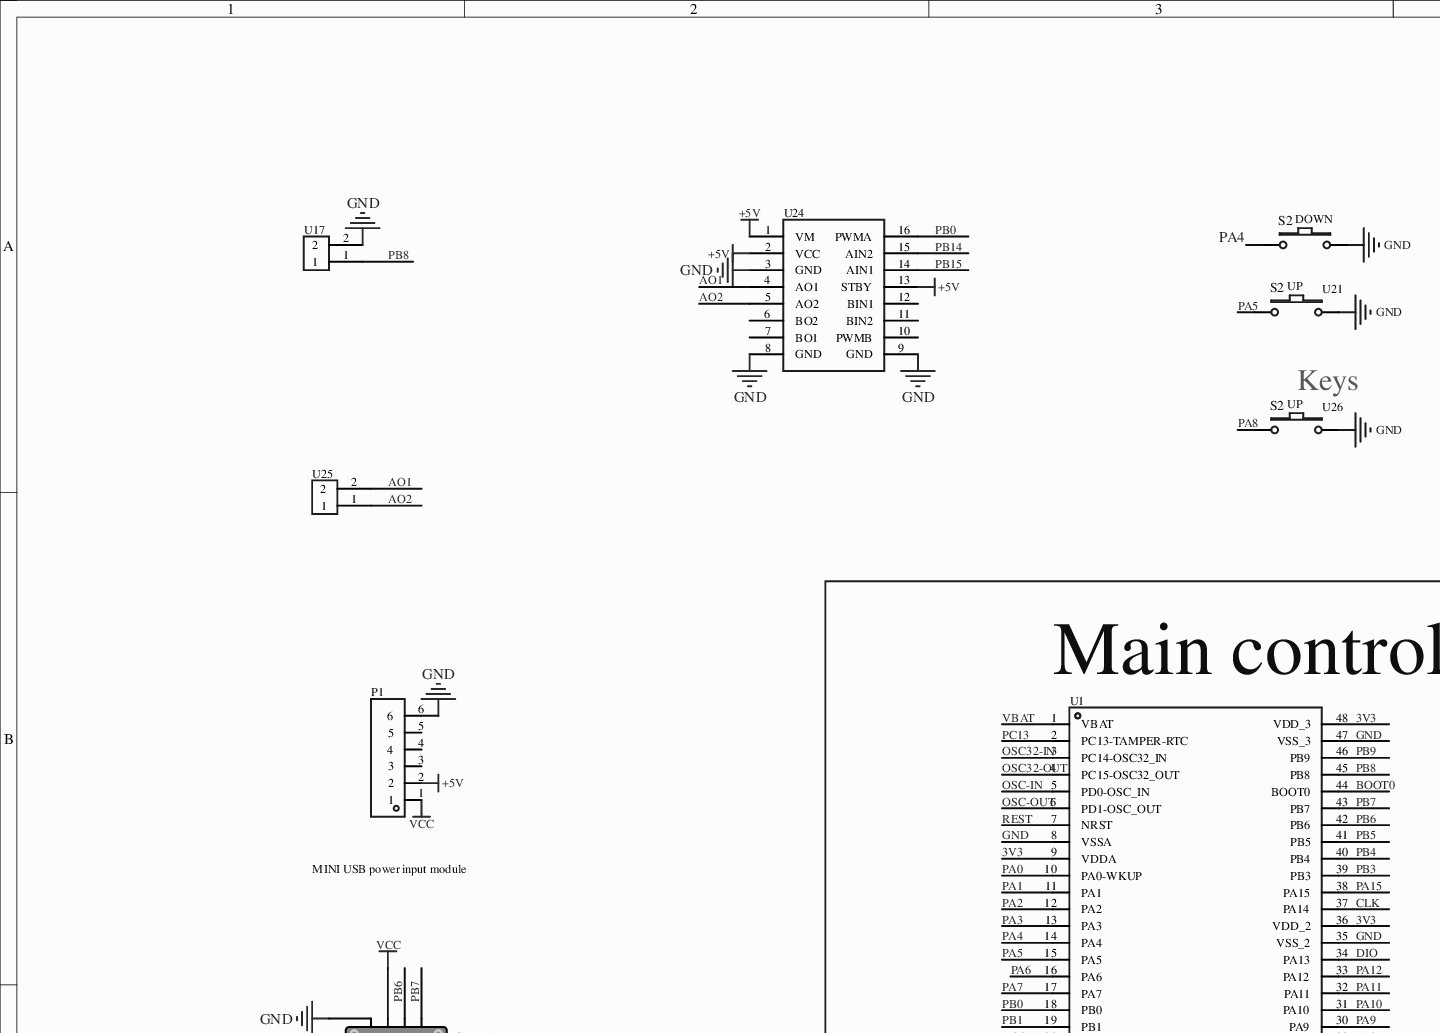
[diagram p0: MISC89131-3.schdoc, top left]
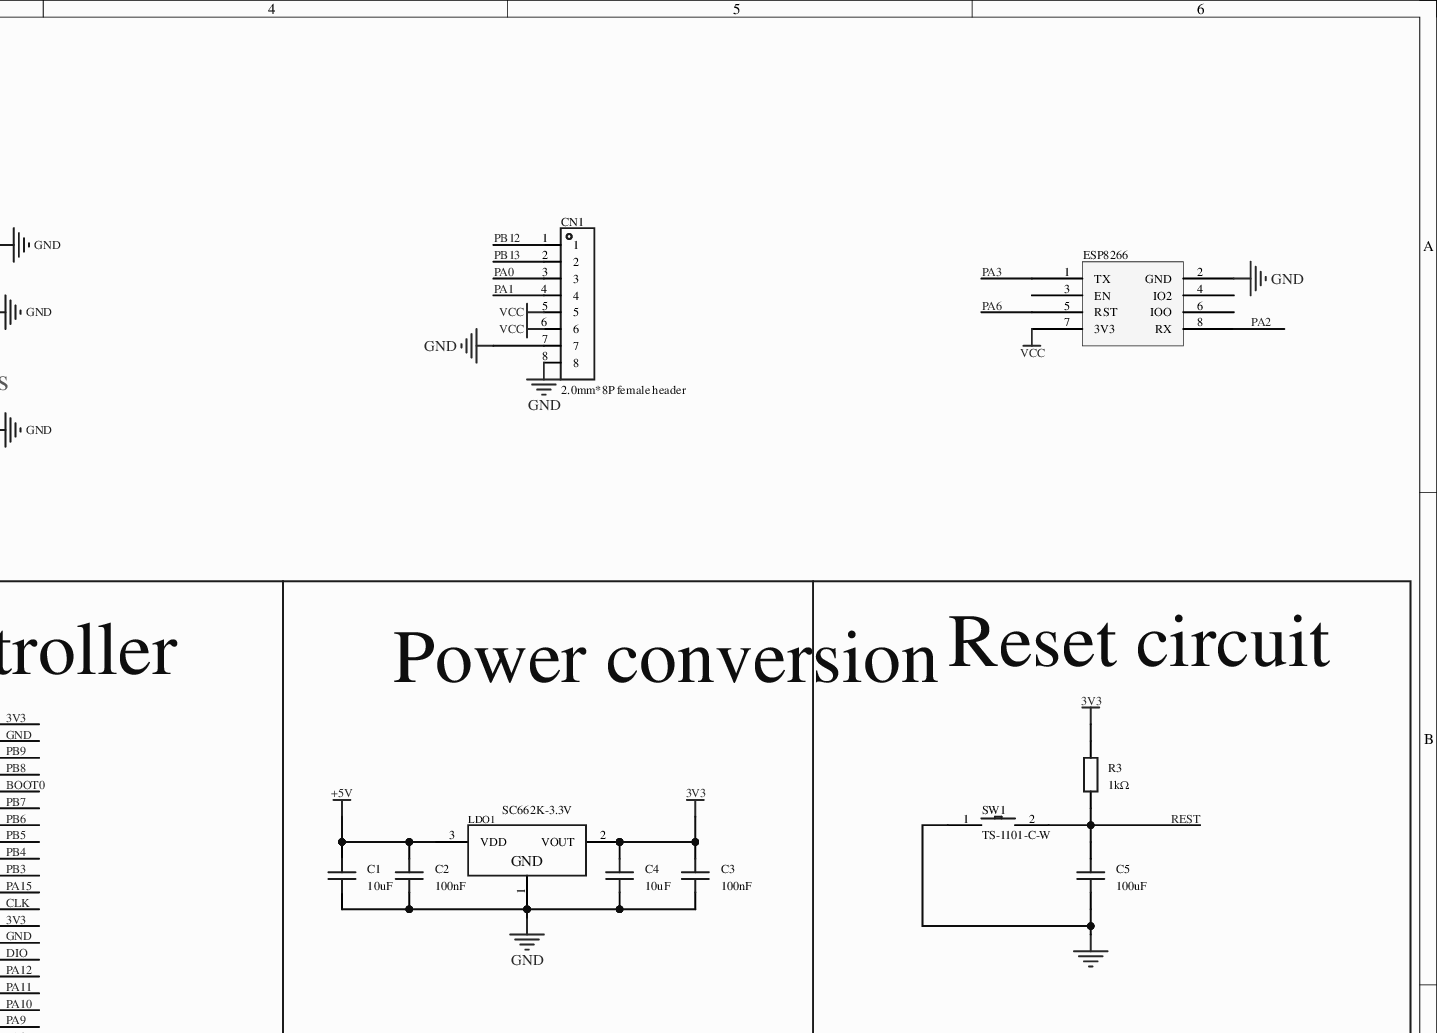
[diagram p1: MISC89131-3.schdoc, top right]
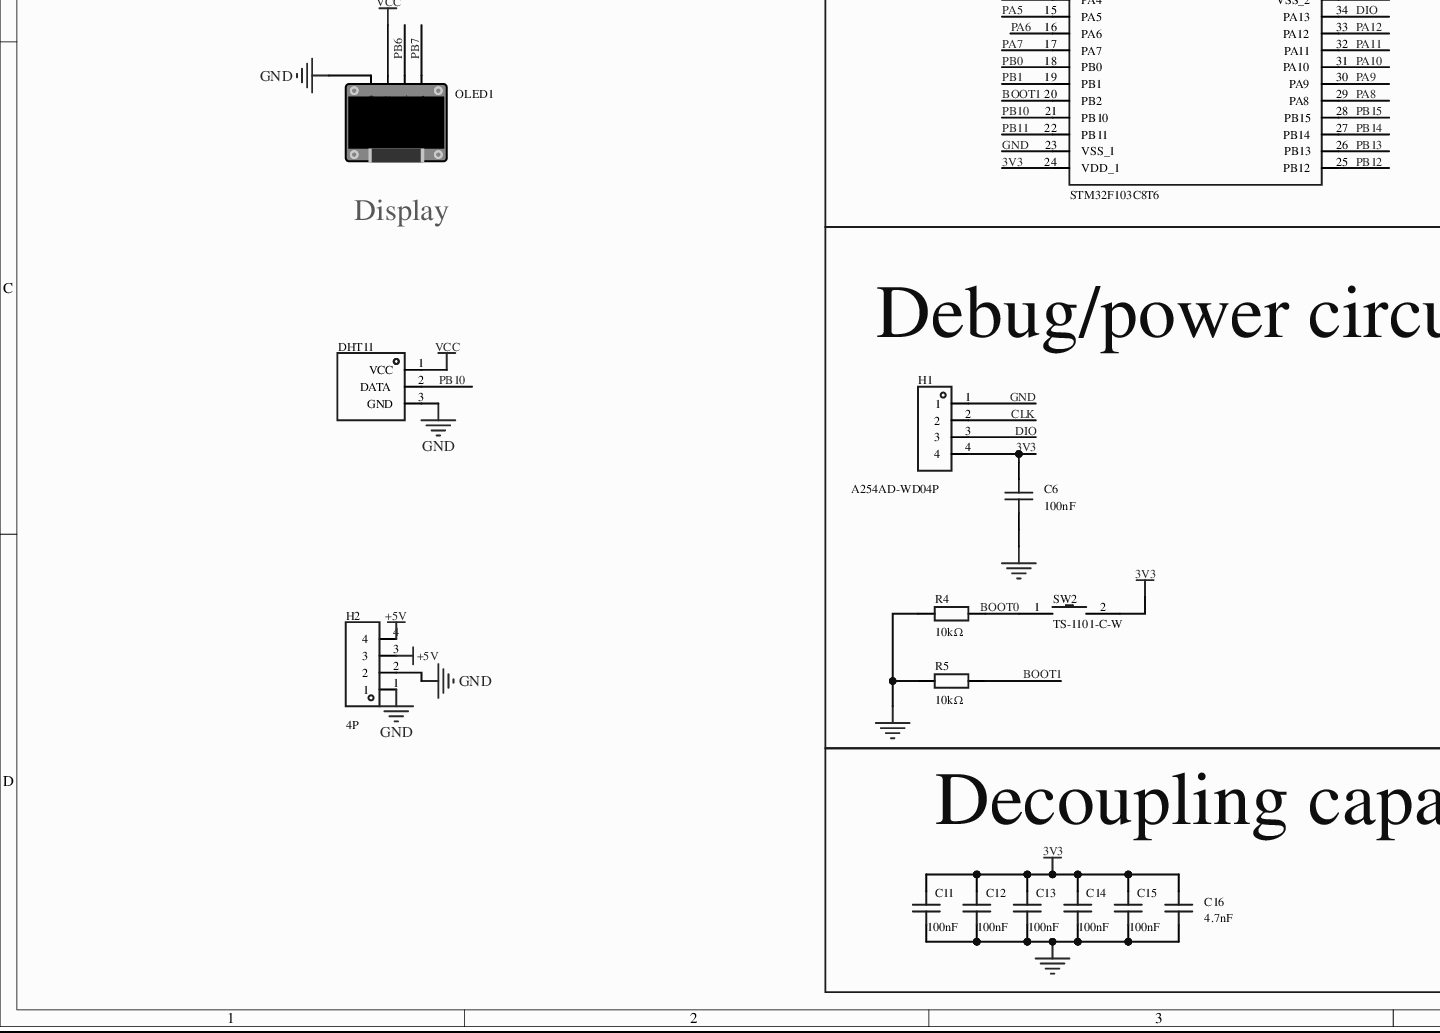
[diagram p2: MISC89131-3.schdoc, bottom left]
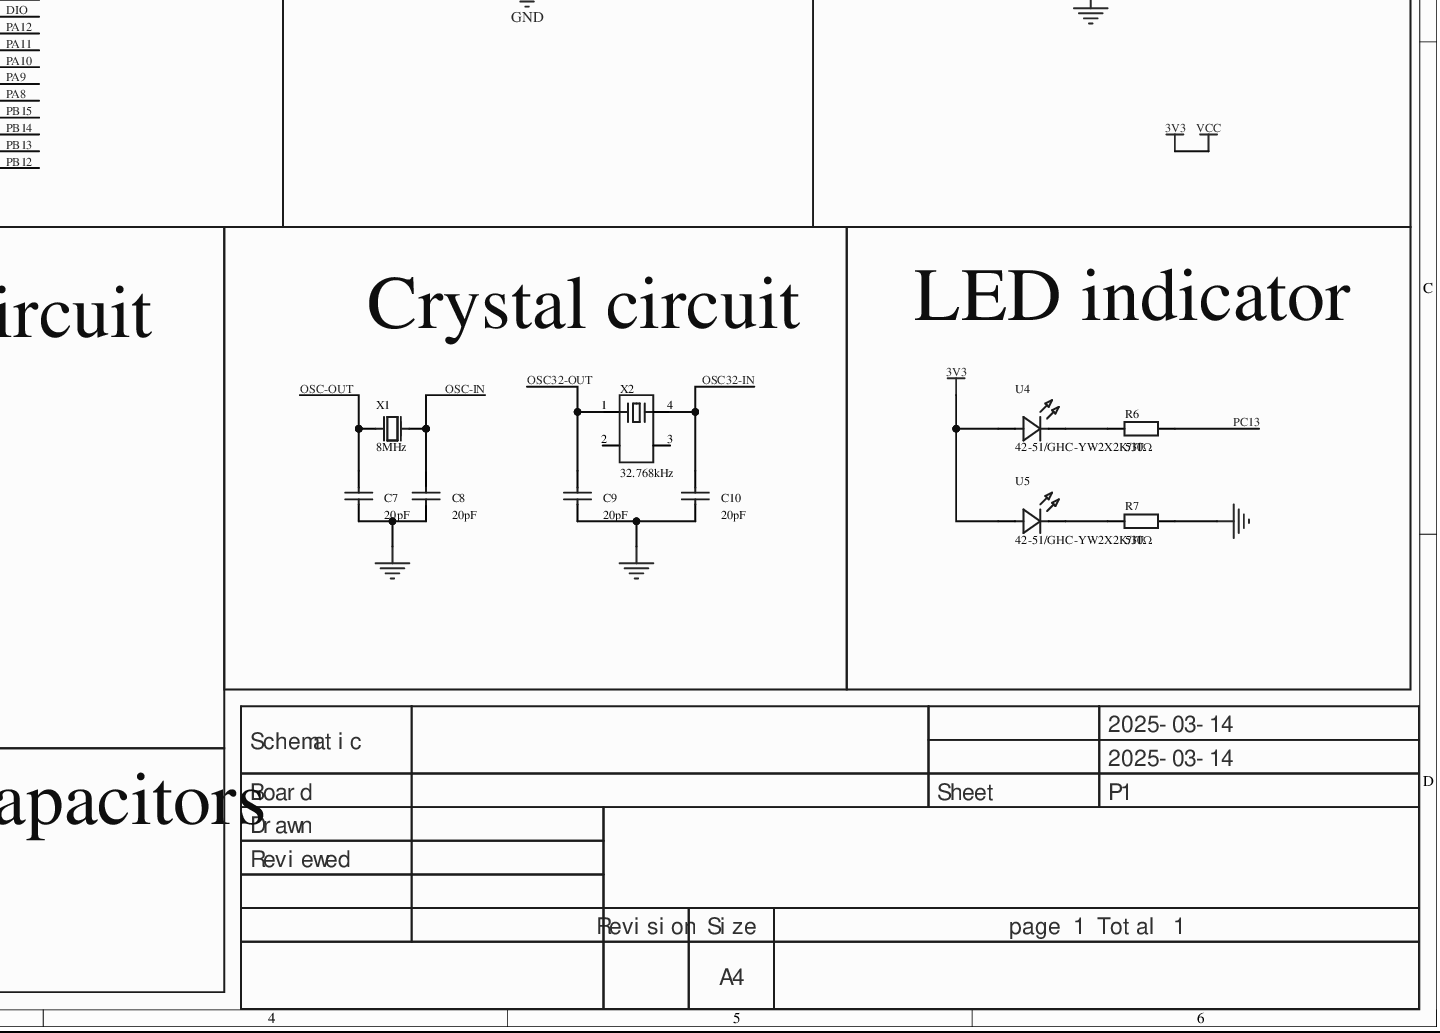
[diagram p3: MISC89131-3.schdoc, bottom right]
# Altium project MISC89131-2.PrjPcb
1 sheet, 42 parts. Net scope: global (net labels, ports and power ports of the same name join across sheets).
Board file: MISC89131.pcbdoc

## Sheet MISC89131-3.schdoc
size 420 x 297 mm; Version: V1.0; @Project Name: MISC89131; @Page Count: 1; @Update Date: 2025-03-14; @Create Date: 2025-03-14; @Schematic Name: MISC89131; @Page No: 1; @Create Time: 21:31:09; @Update Time: 21:31:14; @Board Name: MISC89131

### Parts
C1  10uF  [C0603]
C2  100nF  [C0603]
C3  100nF  [C0603]
C4  10uF  [C0603]
C5  100uF  [C1206]
C6  100nF  [C0603]
C7  20pF  [C0603]
C8  20pF  [C0603]
C9  20pF  [C0603]
C10  20pF  [C0603]
C11  100nF  [C0603]
C12  100nF  [C0603]
C13  100nF  [C0603]
C14  100nF  [C0603]
C15  100nF  [C0603]
C16  4.7nF  [C0603]
CN1  2.0mm*8P female header  [HDR-TH_8P-P1.27_2.0MM-8P]
DHT11  (no value)  [PIN3直插DHT11]
ESP8266  (no value)  [ESP8266-01S_Module]
H1  A254AD-WD04P  [HDR-TH_4P-P2.54-H-M-W10.2]
H2  4P  [HDR-TH_4P-P2.54-V-M-3]
LDO1  SC662K-3.3V  [SOT-23-3_L2.9-W1.3-P1.90-LS2.4-BR]
OLED1  (no value)  [0.96OLED_4P]
P1  MINI USB power input module  [HDR-TH_6P-P2.54-V-F]
R3  1kΩ  [R0603]
R4  10kΩ  [R0603]
R5  10kΩ  [R0603]
R6  510Ω  [R0603]
R7  510Ω  [R0603]
SW1  TS-1101-C-W  [SW-SMD_L6.0-W3.3-LS8.0]
SW2  TS-1101-C-W  [SW-SMD_L6.0-W3.3-LS8.0]
U1  STM32F103C8T6  [LQFP-48_L7.0-W7.0-P0.50-LS9.0-BL]
U4  42-51/GHC-YW2X2K/3T  [LED-SMD_L1.6-W0.8-FD_GREEN-1]
U5  42-51/GHC-YW2X2K/3T  [LED-SMD_L1.6-W0.8-FD_GREEN-1]
U17  (no value)  [2p排针]
U21  UP  [KEY-TH_4P复位按键]
U23  DOWN  [KEY-TH_4P复位按键]
U24  (no value)  [TB6612电机驱动]
U25  (no value)  [2p排针]
U26  UP  [KEY-TH_4P复位按键]
X1  8MHz  [OSC-TH_L10.0-W4.5-P5.00]
X2  32.768kHz  [MC-306_4P-L8.0-W3.2-P5.5-BL]

### Blocks framed on the sheet
Main controller: U1
Power conversion: C1-C4 LDO1
Reset circuit: C5 R3 SW1
Debug/power circuit: C6 H1 R4 R5 SW2
Crystal circuit: C7-C10 X1 X2
LED indicator: R6 R7 U4 U5
Decoupling capacitors: C11-C16

### Nets
3V3: C3.2 C4.2 C6.2 C11.2 C12.2 C13.2 C14.2 C15.2 C16.2 CN1.5 CN1.6 DHT11.1(VCC) ESP8266.7(3V3) H1.4 LDO1.2(VOUT) OLED1.2(VCC) P1.1 R3.2 SW2.2 U1.9(VDDA) U1.24(VDD_1) U1.36(VDD_2) U1.48(VDD_3) U4.1(A) U5.1(A)  [also labelled VCC]
+5V: C1.2 C2.2 H2.3 H2.4 LDO1.3(VDD) P1.2 U24.1(VM) U24.2(VCC) U24.13(STBY)
GND: C1.1 C2.1 C3.1 C4.1 C5.1 C6.1 C7.1 C8.1 C9.1 C10.1 C11.1 C12.1 C13.1 C14.1 C15.1 C16.1 CN1.7 CN1.8 DHT11.3(GND) ESP8266.2(GND) H1.1 H2.1 H2.2 LDO1.1(GND) OLED1.1(GND) P1.6 R4.1 R5.1 R7.2 SW1.1 U1.8(VSSA) U1.23(VSS_1) U1.35(VSS_2) U1.47(VSS_3) U17.2 U21.3 U23.3 U24.3(GND) U24.8(GND) U24.9(GND) U26.3
AO1: U24.4(AO1) U25.2
AO2: U24.5(AO2) U25.1
BOOT0: R4.2 SW2.1 U1.44(BOOT0)
BOOT1: R5.2 U1.20(PB2)
CLK: H1.2 U1.37(PA14)
DIO: H1.3 U1.34(PA13)
OSC32-IN: C10.2 U1.3(PC14-OSC32_IN) X2.4
OSC32-OUT: C9.2 U1.4(PC15-OSC32_OUT) X2.1
OSC-IN: C8.2 U1.5(PD0-OSC_IN) X1.1(OSC1)
OSC-OUT: C7.2 U1.6(PD1-OSC_OUT) X1.2(OSC2)
PA0: CN1.3 U1.10(PA0-WKUP)
PA1: CN1.4 U1.11(PA1)
PA2: ESP8266.8(RX) U1.12(PA2)
PA3: ESP8266.1(TX) U1.13(PA3)
PA4: U1.14(PA4) U23.1
PA5: U1.15(PA5) U21.1
PA6: ESP8266.5(RST) U1.16(PA6)
PA7: U1.17(PA7)
PA8: U1.29(PA8) U26.1
PA9: U1.30(PA9)
PA10: U1.31(PA10)
PA11: U1.32(PA11)
PA12: U1.33(PA12)
PA15: U1.38(PA15)
PB0: U1.18(PB0) U24.16(PWMA)
PB1: U1.19(PB1)
PB3: U1.39(PB3)
PB4: U1.40(PB4)
PB5: U1.41(PB5)
PB6: OLED1.3(SCL) U1.42(PB6)
PB7: OLED1.4(SDA) U1.43(PB7)
PB8: U1.45(PB8) U17.1
PB9: U1.46(PB9)
PB10: DHT11.2(DATA) U1.21(PB10)
PB11: U1.22(PB11)
PB12: CN1.1 U1.25(PB12)
PB13: CN1.2 U1.26(PB13)
PB14: U1.27(PB14) U24.15(AIN2)
PB15: U1.28(PB15) U24.14(AIN1)
PC13: R6.2 U1.2(PC13-TAMPER-RTC)
REST: C5.2 R3.1 SW1.2 U1.7(NRST)
VBAT: U1.1(VBAT)
NetR6_1: R6.1 U4.2(C)
NetR7_1: R7.1 U5.2(C)

Not connected (* = marked no-connect by the designer): ESP8266 3(EN)* 4(IO2)* 6(IOO)*; P1 3* 4* 5*; U24 6(BO2)* 7(BO1)* 10(PWMB)* 11(BIN2)* 12(BIN1)*; X2 2 3

### Notes on the sheet
- Keys
- Display
- 2025-03-14
- Schematic
- Board
- Sheet
- P1
- Drawn
- Reviewed
- Revision
- Size
- A4
- page 1 Total 1

### Library data of the parts
C1 C4 = CL10A106KP8NNNC: Capacitance:10uF;Tolerance:±10%;Rated voltage:10V;Dielectric (temperature coefficient):X5R;; Manufacturer: SAMSUNG(三星); AddInBom: yes; ModelId: ac125912035d415993ca9572d50418b1; ModelName: C0603_L1.6-W0.8-H0.8; ModelTransform: 62.992,31.496,0,0,0,0,0,0,0; Tolerance: ±10%; Voltage Rated: 10V; Temperature Coefficient: X5R; Device: CL10A106KP8NNNC; Symbol: CL10A106KP8NNNC; LCSC Part Name: 10uF ±10% 10V; SupplierPart: C19702; ManufacturerPart: CL10A106KP8NNNC; Supplier Footprint: 0603; JLCPCB Part Class: Basic library; Datasheet: https://example.com/upload/public/pdf/source/20160103/1457707703378.pdf; Supplier: LCSC; ConvertToPcb: yes; FootprintName: C0603; Value: 10uF
C2 C3 = CC0603KRX7R9BB104: Capacitance:100nF;Tolerance:±10%;Rated voltage:50V;Dielectric (temperature coefficient):X7R;; Manufacturer: YAGEO(国巨); AddInBom: yes; ModelId: ac125912035d415993ca9572d50418b1; ModelName: C0603_L1.6-W0.8-H0.8; ModelTransform: 62.992,31.496,0,0,0,0,0,0,0; Tolerance: ±10%; Voltage Rated: 50V; Temperature Coefficient: X7R; Device: CC0603KRX7R9BB104; Symbol: CC0603KRX7R9BB104; LCSC Part Name: 100nF ±10% 50V; SupplierPart: C14663; ManufacturerPart: CC0603KRX7R9BB104; Supplier Footprint: 0603; JLCPCB Part Class: Basic library; Datasheet: https://example.com/upload/public/pdf/source/20180910/C282072_33301C7F631E79921B82A8DAC6BCC5B3.pdf; Supplier: LCSC; ConvertToPcb: yes; FootprintName: C0603; Value: 100nF
C5 = HGC1206R5107M100NSPJ: Capacitance:100uF;Tolerance:±20%;Rated voltage:10V;Dielectric (temperature coefficient):X5R;; Manufacturer: Chinocera(华瓷); AddInBom: yes; ModelId: e4be705b945545a48e666415e3682bd8; ModelName: C1206_L3.2-W1.6-H1.3; ModelTransform: 125.984,62.992,0,0,0,0,0,0,0; Tolerance: ±20%; Voltage Rated: 10V; Temperature Coefficient: X5R; Symbol: HGC1206R5107M100NSPJ; Device: HGC1206R5107M100NSPJ; LCSC Part Name: 100uF ±20% 10V; SupplierPart: C7432784; ManufacturerPart: HGC1206R5107M100NSPJ; Supplier Footprint: 1206; JLCPCB Part Class: Extended library; Datasheet: https://example.com/upload/public/pdf/source/20240320/FAC3FEC40A78BC5CCCE96C232A94D860.pdf; Supplier: LCSC; ConvertToPcb: yes; FootprintName: C1206; Value: 100uF
C6 C11-C15 = CGA0603X7R104K500JT: Capacitance:100nF;Tolerance:±10%;Rated voltage:50V;Dielectric (temperature coefficient):X7R;; Manufacturer: HRE(芯声); AddInBom: yes; ModelId: ac125912035d415993ca9572d50418b1; ModelName: C0603_L1.6-W0.8-H0.8; ModelTransform: 62.992,31.496,0,0,0,0,0,0,0; Tolerance: ±10%; Voltage Rated: 50V; Temperature Coefficient: X7R; Symbol: CGA0603X7R104K500JT; Device: CGA0603X7R104K500JT; LCSC Part Name: 100nF ±10% 50V; SupplierPart: C6119867; ManufacturerPart: CGA0603X7R104K500JT; Supplier Footprint: 0603; JLCPCB Part Class: Extended library; Supplier: LCSC; ConvertToPcb: yes; FootprintName: C0603; Value: 100nF
C7-C10 = CL10C200JB8NNNC: Capacitance:20pF;Tolerance:±5%;Rated voltage:50V;Dielectric (temperature coefficient):C0G;; Manufacturer: SAMSUNG(三星); AddInBom: yes; ModelId: ac125912035d415993ca9572d50418b1; ModelName: C0603_L1.6-W0.8-H0.8; ModelTransform: 62.992,31.496,0,0,0,0,0,0,0; Tolerance: ±5%; Voltage Rated: 50V; Temperature Coefficient: C0G; Symbol: CL10C200JB8NNNC; Device: CL10C200JB8NNNC; LCSC Part Name: 20pF ±5% 50V; SupplierPart: C1648; ManufacturerPart: CL10C200JB8NNNC; Supplier Footprint: 0603; JLCPCB Part Class: Basic library; Datasheet: https://example.com/upload/public/pdf/source/20160218/1457707763339.pdf; Supplier: LCSC; ConvertToPcb: yes; FootprintName: C0603; Value: 20pF
C16 = CGA0603X7R472K500JT: Capacitance:4.7nF;Tolerance:±10%;Rated voltage:50V;Dielectric (temperature coefficient):X7R;; Manufacturer: HRE(芯声); AddInBom: yes; ModelId: ac125912035d415993ca9572d50418b1; ModelName: C0603_L1.6-W0.8-H0.8; ModelTransform: 62.992,31.496,0,0,0,0,0,0,0; Tolerance: ±10%; Voltage Rated: 50V; Temperature Coefficient: X7R; Symbol: CGA0603X7R472K500JT; Device: CGA0603X7R472K500JT; LCSC Part Name: 4.7nF ±10% 50V; SupplierPart: C7503499; ManufacturerPart: CGA0603X7R472K500JT; Supplier Footprint: 0603; JLCPCB Part Class: Extended library; Supplier: LCSC; ConvertToPcb: yes; FootprintName: C0603; Value: 4.7nF
CN1 = 2.0mm*8P排母: AddInBom: yes; ModelId: 95b80f37f95247e9934e1f38a5a0f20e; ModelTransform: 419.6842,70.866,0,0,0,0,0,0,-78.74; Symbol: 2.0MM*8P female header; Device: 2.0mm*8P female header; LCSC Part Name: 2.0mm*8P排母; SupplierPart: C9900006164; ManufacturerPart: 2.0mm*8P排母; Supplier Footprint: TH-8P; JLCPCB Part Class: Extended Part; Supplier: LCSC; ConvertToPcb: yes; FootprintName: HDR-TH_8P-P1.27_2.0MM-8P; ModelName: HDR-TH_8P-P1.27_2.0MM-8P
DHT11 = DHT11: AddInBom: yes; Device: DHT11; ConvertToPcb: yes; SymbolName: DHT11; FootprintName: PIN3 through-hole DHT11
ESP8266 = ESP8266-01S_Module*: ConvertToPcb: yes; Symbol: ESP8266-01S_Module; Device: ESP8266-01S_Module*; AddInBom: yes; FootprintName: ESP8266-01S_Module
H1 = A254AD-WD04P: 插针结构:1x4P;间距:2.54mm;行距:-;圆针/方针:方针;安装类型:弯插;排数:单排;总PIN位数:4P;额定电流:3A;配合针长度:6mm;塑高:2.5mm;工作温度范围:-40℃~+105℃;; Manufacturer: BXCONN(宝讯); AddInBom: yes; ModelId: 8fb77c134dcb46f68fcbe3019b5d6fb5; ModelTransform: 396.0622,401.574,0,0,0,0,0,-187.008,-118.11; Pin Structure: 1x4P; Pitch: 2.54mm; Circluar Pins/Square Pins: Square pins; Current Rating (Max): 3A; Symbol: A254AD-WD04P; Device: A254AD-WD04P; LCSC Part Name: 排针 间距:2.54mm 1x4P 弯插 方针; SupplierPart: C41413850; ManufacturerPart: A254AD-WD04P; Supplier Footprint: 弯插,P=2.54mm; Datasheet: https://example.com/upload/public/pdf/source/20240923/AB9B16B482278D2B379635B0388B4E48.pdf; Supplier: LCSC; ConvertToPcb: yes; FootprintName: HDR-TH_4P-P2.54-H-M-W10.2; ModelName: HDR-TH_4P-P2.54-H-M-W10.2; Row Spacing: -; Mounting Type: Right-angle; Number of Rows: Single row; Number of Pins: 4P; Length of Mating Pin: 6mm; Insulation Height: 2.5mm; Operating Temperature Range: -40℃~+105℃
H2 = 4P排针: ManufacturerPart: SIP4-CON4排针; Symbol: SIP4-CON4 pin header; Device: 4P pin header; AddInBom: yes; ModelId: 8f992ffc0bd944c6961f69f25c8aaa5a; ModelTransform: 400,100,0,0,0,0,0,0,-137.8; LCSC Part Name: SIP4-CON4排针; SupplierPart: C9900002129; Supplier Footprint: SIP-4_2.54X10.16X2.54P; JLCPCB Part Class: Extended Part; Supplier: LCSC; ConvertToPcb: yes; FootprintName: HDR-TH_4P-P2.54-V-M-3; ModelName: HDR-TH_4P-P2.54-V-M-3
LDO1 = SC662K-3.3V: Output type:Fixed;Output polarity:Positive;Max input voltage:6V;Output voltage:3.3V;Output current:250mA;Power supply rejection ratio (PSRR):50dB@(1kHz);; Manufacturer: FM(富满); AddInBom: yes; ModelId: c62791f0466c4ae2a892c056b845b0ca; ModelName: SOT-23-3P_L2.9-W1.3-H1.0-LS2.4-P0.95; ModelTransform: 98.425,114.173,0,180,0,0,0.0005,-0.0005,0; Output Type: Fixed; Number of Outputs: 1; Maximum Input Voltage: 6V; Output Voltage: 3.3V; Dropout Voltage: 38mV@(10mA); Output Current: 250mA; Symbol: SC662K-3.3V; Device: SC662K-3.3V; Supplier: LCSC; Manufacturer Part: SC662K-3.3V; Supplier Part: C83932; JLCPCB Part Class: Extended library; LCSC Part Name: 输入6V 输出3.3V 250mA 停产; Supplier Footprint: SOT-23; Datasheet: https://example.com/upload/public/pdf/source/20161024/1477288576049.pdf; ConvertToPcb: yes; FootprintName: SOT-23-3_L2.9-W1.3-P1.90-LS2.4-BR; Output Polarity: Positive; Power Supply Rejection Ratio (PSRR): 50dB@(1kHz)
OLED1 = 0.96OLED模块_4P: Device: 0.96OLED module_4P; ConvertToPcb: yes; ModelId: 79c000fdb68d45a296c2e9bedf4f9055; ModelTransform: 1393.69792,1318.895,0,0,0,0,0,-560.079,-137.795; AddInBom: yes; SymbolName: 0.96OLED module_4P; FootprintName: 0.96OLED_4P; Supplier Footprint: 插件; ModelName: 0.96OLED_4P
P1 = 2.54-1*6P母: Socket structure:1x6P;Pitch:2.54mm;Row spacing:-;Mounting type:Through-hole;Rows:Single row;Total holes:6P;Plastic height:-;Contact material:-;Contact plating:-;; Manufacturer Part: MINI USB电源输入模块; Manufacturer: BOOMELE(博穆精密); Symbol: Header-Female-2.54_1x6; Device: 2.54-1*6P female header; AddInBom: yes; ModelId: 0f5bcf94dcda47d085f24cdca1696fe9; ModelTransform: 619.684,94.488,0,0,0,0,0,0,-125.984; Holes Structure: 1x6P; Pitch: 2.54mm; Number of Holes: 6P; LCSC Part Name: 间距:2.54mm 1x6P 直插; SupplierPart: C40877; Supplier Footprint: 插件,P=2.54mm; JLCPCB Part Class: Extended library; Datasheet: https://example.com/upload/public/pdf/source/20210301/C2718488_F4427B881E42CAA8DDB0B1C12B3A522C.pdf; Supplier: LCSC; ConvertToPcb: yes; FootprintName: HDR-TH_6P-P2.54-V-F; ModelName: HDR-TH_6P-P2.54-V-F; Row Spacing: -; Mounting Type: Through-hole; Number of Rows: Single row; Insulation Height: -; Contact Material: -; Contact Plating: -
R3 = RC0603FR-071KL: Resistor type:Thick film resistor;Resistance:1kΩ;Tolerance:±1%;Power:100mW;Max working voltage:75V;Temperature coefficient:±100ppm/℃;; Manufacturer: YAGEO(国巨); AddInBom: yes; ModelId: fc143cca1e79419f9cd78b61e9279f08; ModelTransform: 31.8897,63.7794,0,90,0,0,0,0,0; Tolerance: ±1%; Power(Watts): 100mW; Overload Voltage (Max): 75V; Symbol: RC0603FR-071KL; Device: RC0603FR-071KL; LCSC Part Name: 厚膜电阻 1kΩ ±1% 100mW; SupplierPart: C22548; ManufacturerPart: RC0603FR-071KL; Supplier Footprint: 0603; JLCPCB Part Class: Extended library; Datasheet: https://example.com/upload/public/pdf/source/20180316/70C0E2BDAE7FCC62C531A5A58D202EE1.pdf; Supplier: LCSC; ConvertToPcb: yes; FootprintName: R0603; ModelName: R0603; Type: Thick film resistor; Value: 1kΩ; Temperature Coefficient: ±100ppm/℃; Operating Temperature Range: -55℃~+155℃
R4 R5 = 0603WAF1002T5E: Resistor type:Thick film resistor;Resistance:10kΩ;Tolerance:±1%;Power:100mW;Max working voltage:75V;Temperature coefficient:±100ppm/℃;; Manufacturer: UNI-ROYAL(厚声); AddInBom: yes; ModelId: fc143cca1e79419f9cd78b61e9279f08; ModelTransform: 31.8897,63.7794,0,90,0,0,0,0,0; Tolerance: ±1%; Power(Watts): 100mW; Overload Voltage (Max): 75V; Symbol: 0603WAF1002T5E; Device: 0603WAF1002T5E; LCSC Part Name: 厚膜电阻 10kΩ ±1% 100mW; SupplierPart: C25804; ManufacturerPart: 0603WAF1002T5E; Supplier Footprint: 0603; JLCPCB Part Class: Basic library; Datasheet: https://example.com/upload/public/pdf/source/20200306/C422600_1E6D84923E4A46A82E41ADD87F860B5C.pdf; Supplier: LCSC; ConvertToPcb: yes; FootprintName: R0603; ModelName: R0603; Type: Thick film resistor; Value: 10kΩ; Temperature Coefficient: ±100ppm/℃; Operating Temperature Range: -55℃~+155℃
R6 R7 = 0603WAF5100T5E: Resistor type:Thick film resistor;Resistance:510Ω;Tolerance:±1%;Power:100mW;Max working voltage:75V;Temperature coefficient:±100ppm/℃;; Manufacturer: UNI-ROYAL(厚声); AddInBom: yes; ModelId: fc143cca1e79419f9cd78b61e9279f08; ModelTransform: 31.8897,63.7794,0,90,0,0,0,0,0; Tolerance: ±1%; Power(Watts): 100mW; Overload Voltage (Max): 75V; Symbol: 0603WAF5100T5E; Device: 0603WAF5100T5E; LCSC Part Name: 510Ω ±1% 100mW 厚膜电阻; SupplierPart: C23193; ManufacturerPart: 0603WAF5100T5E; Supplier Footprint: 0603; JLCPCB Part Class: Basic library; Datasheet: https://example.com/upload/public/pdf/source/20200306/C422600_1E6D84923E4A46A82E41ADD87F860B5C.pdf; Supplier: LCSC; ConvertToPcb: yes; FootprintName: R0603; ModelName: R0603; Type: Thick film resistor; Value: 510Ω; Temperature Coefficient: ±100ppm/℃; Operating Temperature Range: -55℃~+155℃
SW1 SW2 = TS-1101-C-W: 电路结构:单刀单掷;按钮形状:矩形按钮;作用力:260gf;安装方式:立贴;开关长度:6mm;开关宽度:3.6mm;开关高度:2.5mm;带支架:不带;触点电流:50mA;额定电压(AC):-;额定电压(DC):12V;额定功率:-;绝缘电阻:-;带灯:无;机械寿命:5万次;; Manufacturer: XKB Connectivity(中国星坤); AddInBom: yes; ModelId: b2f4ea9f0afc4b0786d53dba66ceb9e4; ModelName: SW-SMD_L6.0-W3.3-H5-LS8.0; ModelTransform: 314.96,129.921,0,0,0,0,0,0,0; Circuit: SPST; Actuator Style: Rectangular button; Operating Force: 260gf; Switch Length: 6mm; Switch Width: 3.6mm; Switch Height: 2.5mm; Strike Gundam: No; Contact Current: 50mA; Voltage Rating (DC): 12V; Actuator/Cap Color: White with light green tint; With Lamp: None; Mechanical Life: 5 ten-thousand cycles; Symbol: TS-1101-C-W; Device: TS-1101-C-W; LCSC Part Name: 6*3.6*2.5mm 立贴 轻触开关; SupplierPart: C318938; ManufacturerPart: TS-1101-C-W; Supplier Footprint: SMD; JLCPCB Part Class: Extended library; Datasheet: https://example.com/upload/public/pdf/source/20200227/C318938_C2E53B1EEDE37D980A33616AC086DE53.pdf; Supplier: LCSC; ConvertToPcb: yes; FootprintName: SW-SMD_L6.0-W3.3-LS8.0; Mounting Style: Surface mount; Voltage Rating (AC): -; Power Rating: -; Insulation Resistance: -; IP Rating: -; Pin Style: -; Operating Temperature: -30℃~+85℃
U1 = STM32F103C8T6: CPU内核:ARM-M3;程序存储容量:64KB;RAM总容量:20KB;GPIO端口数量:37;工作电压范围:2V~3.6V;CPU最大主频:72MHz;程序存储器类型:FLASH;; Manufacturer: ST(意法半导体); AddInBom: yes; ModelId: 093be70396ff421eb2cdb946d5311efc; ModelName: LQFP-48_L7.0-W7.0-H1.4-LS9.0-P0.50; ModelTransform: 354.331,354.331,0,0,0,0,0,0,0; CPU Core: ARM-M3; Program Storage Size: 64KB; RAM Size: 20KB; GPIO Ports Number: 37; CPU Maximum Speed: 72MHz; Program Memory Type: FLASH; ADC (Bit): 12bit; Peripheral/Function: Watchdog; DMA; Watchdog; Temperature sensor; Symbol: STM32F103C8T6; Device: STM32F103C8T6; LCSC Part Name: 主流增强型ARM Cortex-M3 MCU，具有64 KB Flash、72 MHz CPU、电机控制、USB和CAN; SupplierPart: C8734; ManufacturerPart: STM32F103C8T6; Supplier Footprint: LQFP-48(7x7); JLCPCB Part Class: Extended library; Datasheet: https://example.com/upload/public/pdf/source/20220812/8363ACEC51AD55ECEB84799464F7CB85.pdf; Supplier: LCSC; ConvertToPcb: yes; FootprintName: LQFP-48_L7.0-W7.0-P0.50-LS9.0-BL; Operating Voltage Range: 2V~3.6V; Operating Temperature Range: -40℃~+85℃; DAC (Bit): -; PWM (Bit): -; Universal Serial Bus: Yes; Internal Comparator: -; communication protocol: -; Watchdog: Yes; Real-Time Clock: -; Infrared Data Association: Yes; Low-Voltage Detect: Yes; CCP Capture/Compare: -; Secure Digital Input and Output: -; Direct Memory Access: Yes; Internal Oscillator: Yes
U4 U5 = 42-51/GHC-YW2X2K/3T: Emitted color:Emerald green;Forward current:-;Dominant wavelength:520nm~535nm;Luminous intensity:2850mcd;; Manufacturer: EVERLIGHT(亿光); AddInBom: yes; ModelId: feee2acead2344579596fed70e7e7f0f; ModelTransform: 63.7794,31.89954,0,0,0,0,0,0,0; Symbol: 42-51/GHC-YW2X2K/3T; Device: 42-51/GHC-YW2X2K/3T; LCSC Part Name: 正发光贴片灯 颜色正绿色 发光二极管; SupplierPart: C5136797; ManufacturerPart: 42-51/GHC-YW2X2K/3T; Supplier Footprint: 0603; JLCPCB Part Class: Extended library; Datasheet: https://example.com/upload/public/pdf/source/20220916/FBE88CF67A3FC292A254CF6ACE30EBDE.pdf; Supplier: LCSC; ConvertToPcb: yes; FootprintName: LED-SMD_L1.6-W0.8-FD_GREEN-1; ModelName: LED-SMD_L1.6-W0.8-FD_GREEN-1; Emitted Color: Emerald green; Forward Current: -; Dominant Wavelength: 520nm~535nm; Luminous Intensity: 2850mcd
U17 U25 = 2p排针: Device: 2p pin header; AddInBom: yes; ConvertToPcb: yes; SymbolName: 2p pin header; FootprintName: 2p pin header
U21 U23 U26 = 按键4P: Origin Footprint: KEY-TH_4P reset button; Device: 4P button; Convert to PCB: yes; Symbol: 4P button; Add into BOM: yes; FootprintName: KEY-TH_4P reset button
U24 = TB6612: ConvertToPcb: yes; ModelId: d5a115ce26e344c09903b50ed7d72ae5user; ModelName: TB6612FNG; ModelTransform: 140.5,825.98,822.98,0,0,270,559.06,0,78.74; Symbol: TB6612; Device: TB6612; AddInBom: yes; FootprintName: TB6612 motor driver
X1 = X49SD8MSD2SC: Crystal type:Through-hole crystal;Frequency:8MHz;Frequency tolerance (room temperature):±20ppm;Load capacitance:20pF;Frequency stability (full temperature):±30ppm;; Manufacturer: YXC(扬兴晶振); AddInBom: yes; ModelId: a8e34f6c394c4d60ace7720f62d1ccdf; ModelName: HC-49US_L11.0-W4.5-H3.5-P4.88; ModelTransform: 432.46488,177.165,0,90,0,0,0,0,-137.795; Normal temperature Frequency Tolerance: ±20ppm; External load capacitor: 20pF; Frequency Stability(Full temperature range): ±30ppm; Symbol: X49SD8MSD2SC; Device: X49SD8MSD2SC; LCSC Part Name: 8MHz ±20ppm 20pF; SupplierPart: C21263; ManufacturerPart: X49SD8MSD2SC; Supplier Footprint: HC-49S; JLCPCB Part Class: Extended library; Datasheet: https://example.com/upload/public/pdf/source/20240329/977D7F2434F98B2BE33270BB9FF3D86D.pdf; Supplier: LCSC; ConvertToPcb: yes; FootprintName: OSC-TH_L10.0-W4.5-P5.00; Crystal Type: Through-hole crystal; Value: 8MHz; Operating Temperature: -20℃~+70℃
X2 = Q13MC30610003: Crystal type:SMD crystal;Frequency:32.768kHz;Frequency tolerance (room temperature):±20ppm;Load capacitance:12.5pF;; Manufacturer: EPSON(爱普生); Symbol: Q13MC3061000300; AddInBom: yes; ModelId: 916dfeb1bef54ad28f6513dfe81e803a; ModelName: MC-306_4P-L8.0-W3.2-H2.4-LS3.8-P5.5; ModelTransform: 314.96,149.606,0,0,0,0,0,0,0; Normal temperature Frequency Tolerance: ±20ppm; External load capacitor: 12.5pF; Equivalent Series Resistance (ESR): 35kΩ; Device: Q13MC30610003; LCSC Part Name: 32.768kHz ±20ppm 12.5pF; SupplierPart: C16320; ManufacturerPart: Q13MC30610003; Supplier Footprint: MC-306; JLCPCB Part Class: Extended library; Datasheet: https://example.com/upload/public/pdf/source/20161110/1478747315604.pdf; Supplier: LCSC; ConvertToPcb: yes; FootprintName: MC-306_4P-L8.0-W3.2-P5.5-BL; Crystal Type: SMD crystal; Value: 32.768kHz; Operating Temperature: -40℃~+85℃